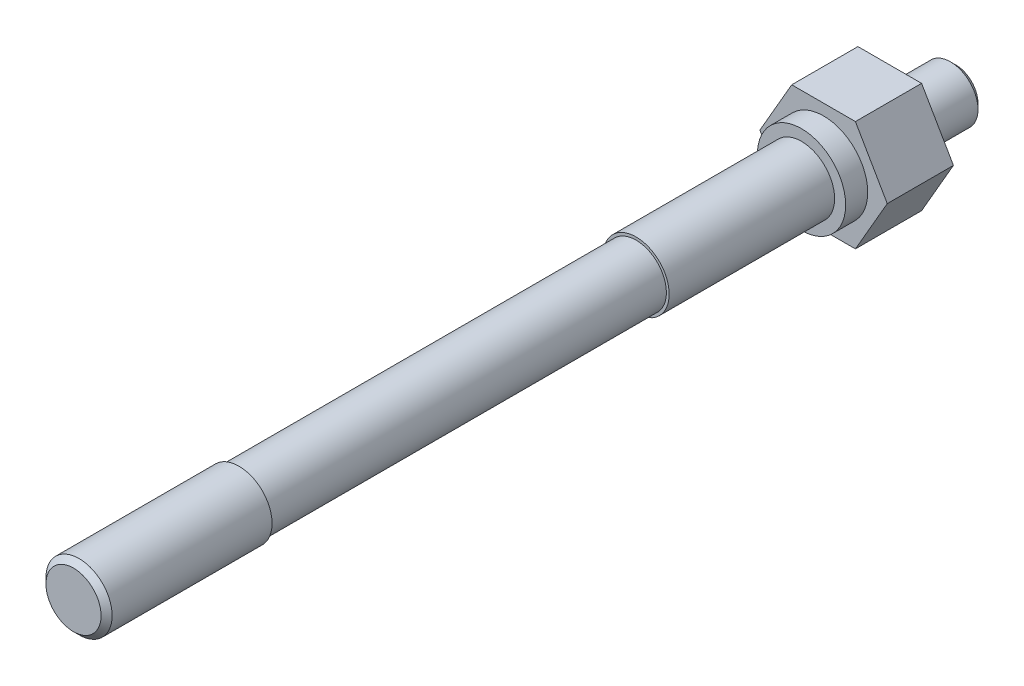
from build123d import *

# Parameters (mm, degrees)
BOSS_EXTRUDE1_DEPTH = 6
SKETCH2_R           = 2.5
BOSS_EXTRUDE2_DEPTH = 6
SKETCH3_R           = 4
BOSS_EXTRUDE3_DEPTH = 2
SKETCH4_R           = 3
BOSS_EXTRUDE4_DEPTH = 66
CHAMFER1_SIZE       = 0.5
SKETCH5_W           = 5
SKETCH5_H           = 36
CHAMFER2_SIZE       = 0.5


with BuildPart() as part:
    # Sketch1 → Boss-Extrude1 (new body)
    with BuildSketch(Plane.XY):
        Polygon((5.773502692, 0), (2.886751346, 5), (-2.886751346, 5), (-5.773502692, 0), (-2.886751346, -5), (2.886751346, -5), align=None)
    extrude(amount=BOSS_EXTRUDE1_DEPTH)

    # Sketch2 → Boss-Extrude2 (add)
    with BuildSketch(Plane(origin=(0, 0, 0), x_dir=(-1, 0, 0), z_dir=(0, 0, -1))):
        with Locations(Location((0, 0, 0), (0, 0, 180))):
            Circle(SKETCH2_R)
    extrude(amount=BOSS_EXTRUDE2_DEPTH)

    # Sketch3 → Boss-Extrude3 (add)
    with BuildSketch(Plane.XY.offset(6)):
        Circle(SKETCH3_R)
    extrude(amount=BOSS_EXTRUDE3_DEPTH)

    # Sketch4 → Boss-Extrude4 (add)
    with BuildSketch(Plane.XY.offset(8)):
        Circle(SKETCH4_R)
    extrude(amount=BOSS_EXTRUDE4_DEPTH)

    # Chamfer1
    chamfer1_edges = [part.edges().sort_by_distance(p)[0] for p in [
        (-3, 0, 74),
    ]]
    chamfer(chamfer1_edges, length=CHAMFER1_SIZE)

    # Sketch5 → Cut-Revolve1 (revolve, cut)
    with BuildSketch(Plane(origin=(0, 0, 0), x_dir=(1, 0, 0), z_dir=(0, 1, 0))):
        with Locations((5.25, -41)):
            Rectangle(SKETCH5_W, SKETCH5_H)
    revolve(axis=Axis((0, 0, 73.5), (0, 0, -1)), mode=Mode.SUBTRACT)

    # Chamfer2
    chamfer2_edges = [part.edges().sort_by_distance(p)[0] for p in [
        (-2.5, 0, -6),
    ]]
    chamfer(chamfer2_edges, length=CHAMFER2_SIZE)


solid = part.part
